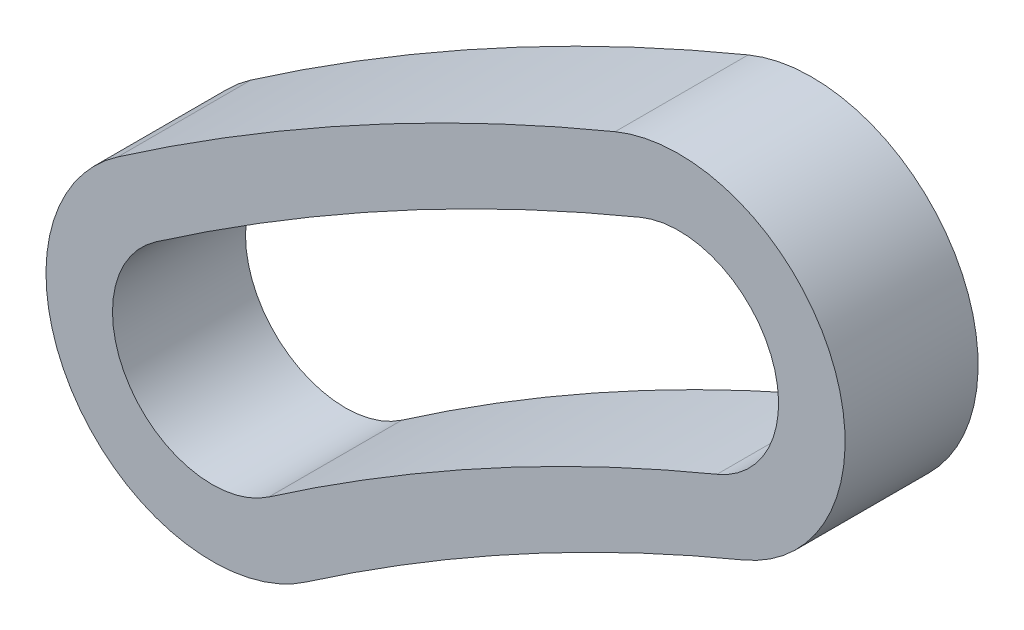
SolidWorks part; units mm, degrees
ref_plane "Front Plane" through (0, 0, 0) normal (0, 0, 1) x (1, 0, 0)
ref_plane "Top Plane" through (0, 0, 0) normal (0, 1, 0) x (1, 0, 0)
ref_plane "Right Plane" through (0, 0, 0) normal (1, 0, 0) x (0, 0, -1)
other "Configuration Table"
sketch "Sketch2" plane through (0, 0, 0) normal (0, 0, 1) x (1, 0, 0)
  arc A0 (-399.3896, 339.1859) -> (-364.3142, 358.2599) centre (-291.5852, 182.7307) cw construction
  arc A1 (-367.1851, 365.1887) -> (-403.645, 345.3617) centre (-291.5852, 182.7307) ccw
  arc A2 (-361.4433, 351.3311) -> (-395.1341, 333.01) centre (-291.5852, 182.7307) ccw
  arc A3 (-361.4433, 351.3311) -> (-367.1851, 365.1887) centre (-364.3142, 358.2599) ccw
  arc A4 (-403.645, 345.3617) -> (-395.1341, 333.01) centre (-399.3896, 339.1859) ccw
  arc A5 (-369.099, 369.8079) -> (-406.482, 349.479) centre (-291.5852, 182.7307) ccw
  arc A6 (-406.482, 349.479) -> (-392.2972, 328.8928) centre (-399.3896, 339.1859) ccw
  arc A7 (-359.5294, 346.7119) -> (-392.2972, 328.8928) centre (-291.5852, 182.7307) ccw
  arc A8 (-359.5294, 346.7119) -> (-369.099, 369.8079) centre (-364.3142, 358.2599) ccw
  point P3 (-382.3543, 349.6468)
  dimension "D1" = 7.5
  dimension "D2" = 190
  dimension "D3" = 5
extrude "Boss-Extrude1" add sketch "Sketch2" along normal blind 10
